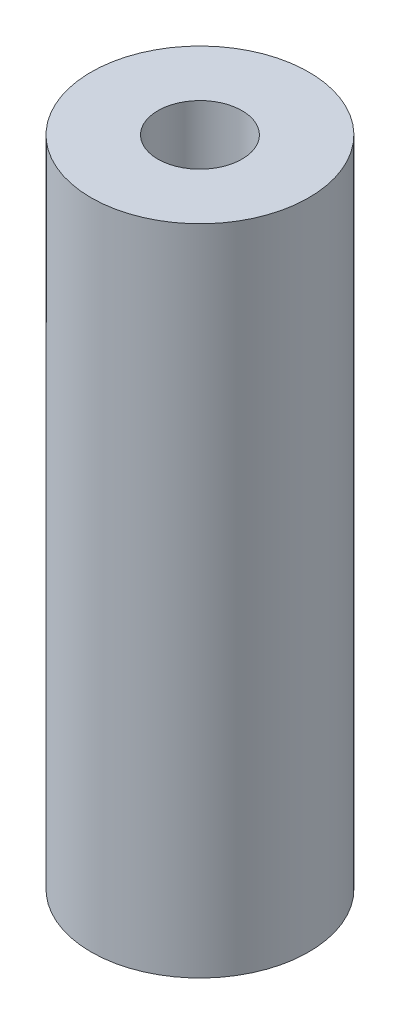
from build123d import *

# Parameters (mm, degrees)
SKETCH1_R              = 11
BOSS_EXTRUDE1_DEPTH    = 66
M10_TAPPED_HOLE1_D     = 8.5
M10_TAPPED_HOLE1_DEPTH = 25
M10_TAPPED_HOLE1_TIP   = 2.553657631


with BuildPart() as part:
    # Sketch1 → Boss-Extrude1 (new body)
    with BuildSketch(Plane(origin=(0, 0, 0), x_dir=(1, 0, 0), z_dir=(0, 1, 0))):
        with Locations(Location((0, 0, 0), (0, 0, 270))):
            Circle(SKETCH1_R)
    extrude(amount=BOSS_EXTRUDE1_DEPTH)

    # M10 Tapped Hole1
    with Locations(Plane(origin=(0, 66, 0), x_dir=(1, 0, 0), z_dir=(0, 1, 0))):
        with Locations((0, 0)):
            Hole(M10_TAPPED_HOLE1_D / 2, depth=M10_TAPPED_HOLE1_DEPTH)
            with Locations((0, 0, -(M10_TAPPED_HOLE1_DEPTH + M10_TAPPED_HOLE1_TIP / 2))):  # 118° drill point
                Cone(0, M10_TAPPED_HOLE1_D / 2, M10_TAPPED_HOLE1_TIP, mode=Mode.SUBTRACT)


solid = part.part
